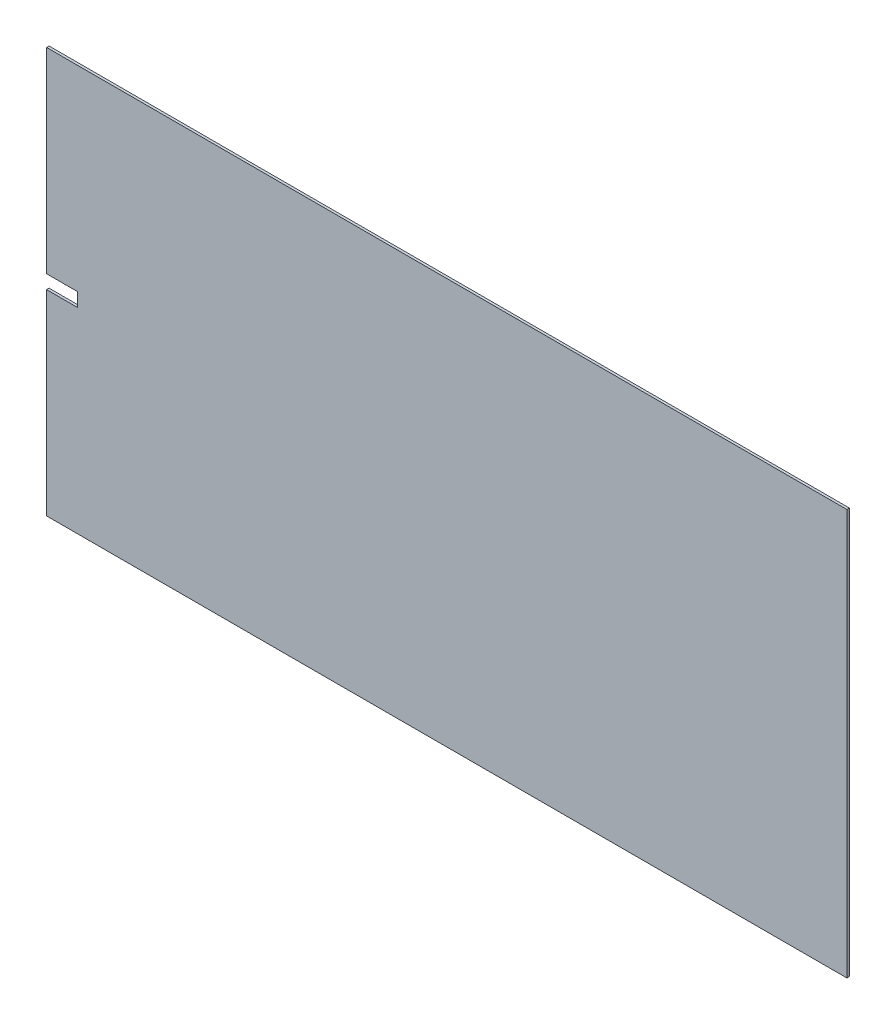
SolidWorks part; units mm, degrees
material "Q235"
ref_plane "Front Plane" through (0, 0, 0) normal (0, 0, 1) x (1, 0, 0)
ref_plane "Top Plane" through (0, 0, 0) normal (0, 1, 0) x (1, 0, 0)
ref_plane "Right Plane" through (0, 0, 0) normal (1, 0, 0) x (0, 0, -1)
sketch "Sketch1" plane through (0, 0, 0) normal (0, 0, 1) x (1, 0, 0)
  line L0 (0, 315) -> (50, 315)
  line L1 (0, 0) -> (1286, 0)
  line L2 (0, 0) -> (0, 315)
  line L3 (0, 652) -> (1286, 652)
  line L4 (1286, 0) -> (1286, 652)
  line L5 (50, 315) -> (50, 337)
  line L6 (50, 337) -> (0, 337)
  line L7 (0, 337) -> (0, 652)
  dimension "D1" = 1286
  dimension "D2" = 652
  dimension "D3" = 50
  dimension "D4" = 22
  dimension "D5" = 315
extrude "Boss-Extrude1" add sketch "Sketch1" along normal blind 4
